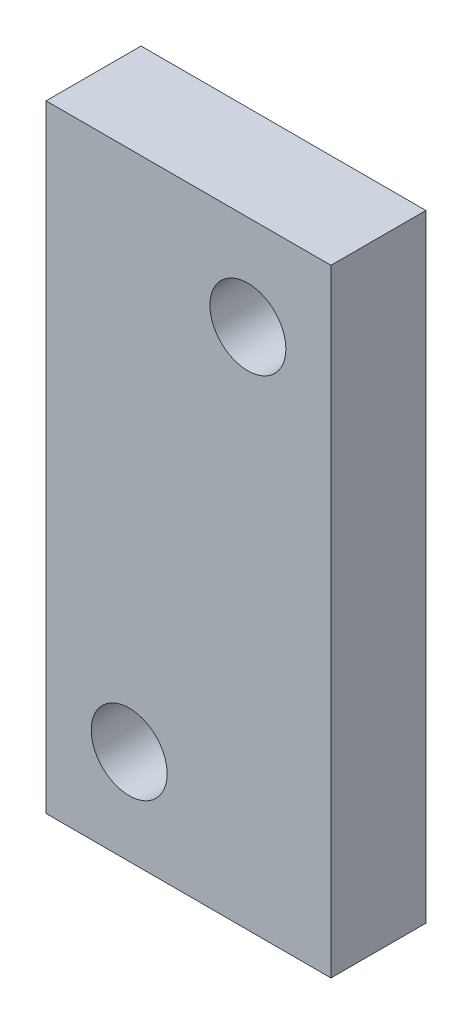
from build123d import *

# Parameters (mm, degrees)
SKETCH_1_W          = 24
SKETCH_1_H          = 52
EXTRUDE_1_DEPTH     = 4
SKETCH_2_R          = 3.2
CUT_EXTRUDE_1_DEPTH = 14


with BuildPart() as part:
    # 草图1 → 凸台-拉伸1 (new, symmetric)
    with BuildSketch(Plane.XY):
        Rectangle(SKETCH_1_W, SKETCH_1_H)
    extrude(amount=EXTRUDE_1_DEPTH, both=True)

    # 草图2 → 切除-拉伸1 (cut, symmetric)
    with BuildSketch(Plane.XY):
        with Locations((-5, -18)):
            Circle(SKETCH_2_R)
        with Locations((5, 18)):
            Circle(SKETCH_2_R)
    extrude(amount=CUT_EXTRUDE_1_DEPTH, both=True, mode=Mode.SUBTRACT)


solid = part.part
